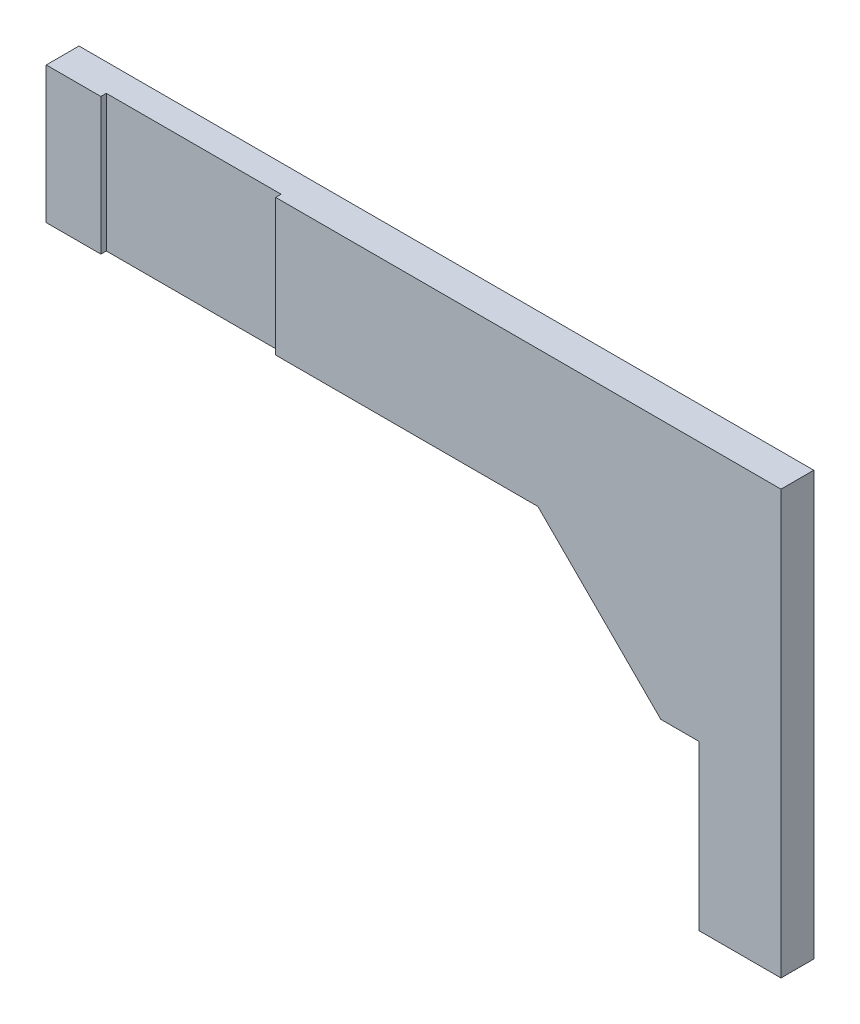
from build123d import *

# Parameters (mm, degrees)
EXTRUDE_1_DEPTH     = 6
SKETCH_2_W          = 64
SKETCH_2_H          = 50
CUT_EXTRUDE_1_DEPTH = 2


with BuildPart() as part:
    # 草图1 → 凸台-拉伸1 (new, symmetric)
    with BuildSketch(Plane.XY):
        Polygon((0, 0), (0, 60), (-14, 60), (-59, 105), (-239, 105), (-239, 155), (30, 155), (30, 0), align=None)
    extrude(amount=EXTRUDE_1_DEPTH, both=True)

    # 草图2 → 切除-拉伸1 (cut)
    with BuildSketch(Plane(origin=(0, 0, 6), x_dir=(-1, 0, 0), z_dir=(0, 0, -1))):
        with Locations((187, 130)):
            Rectangle(SKETCH_2_W, SKETCH_2_H)
    extrude(amount=CUT_EXTRUDE_1_DEPTH, mode=Mode.SUBTRACT)


solid = part.part
